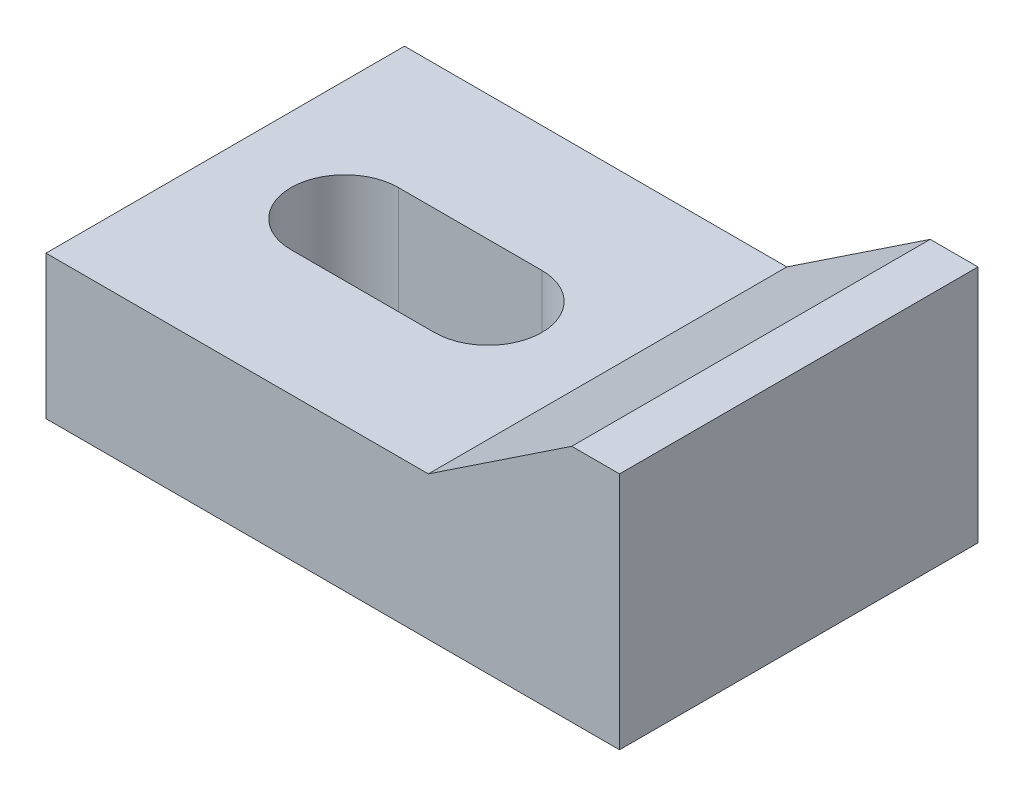
from build123d import *

# Parameters (mm, degrees)
BOSS_EXTRUDE1_DEPTH = 7.5
CUT_EXTRUDE1_REACH  = 17.37


with BuildPart() as part:
    # Sketch1 → Boss-Extrude1 (new, symmetric)
    with BuildSketch(Plane.XY):
        Polygon((4, 1), (-12, 1), (-12, -5), (12, -5), (12, 5), (10, 5), align=None)
    extrude(amount=BOSS_EXTRUDE1_DEPTH, both=True)

    # Sketch2 → Cut-Extrude1 (cut, up to next)
    with BuildSketch(Plane(origin=(0, 1, 0), x_dir=(1, 0, 0), z_dir=(0, 1, 0)), mode=Mode.PRIVATE) as cut_extrude1_sk1:
        with BuildLine():
            Line((-7, 2.25), (-1, 2.25))
            ThreePointArc((-1, 2.25), (1.25, 0), (-1, -2.25))
            Line((-1, -2.25), (-7, -2.25))
            ThreePointArc((-7, -2.25), (-9.25, 0), (-7, 2.25))
        make_face()
    cut_extrude1_tool1 = extrude(cut_extrude1_sk1.sketch, amount=-CUT_EXTRUDE1_REACH, mode=Mode.PRIVATE) & part.part
    add(cut_extrude1_tool1.solids().sort_by_distance((-4, 1, 0))[0], mode=Mode.SUBTRACT)


solid = part.part
